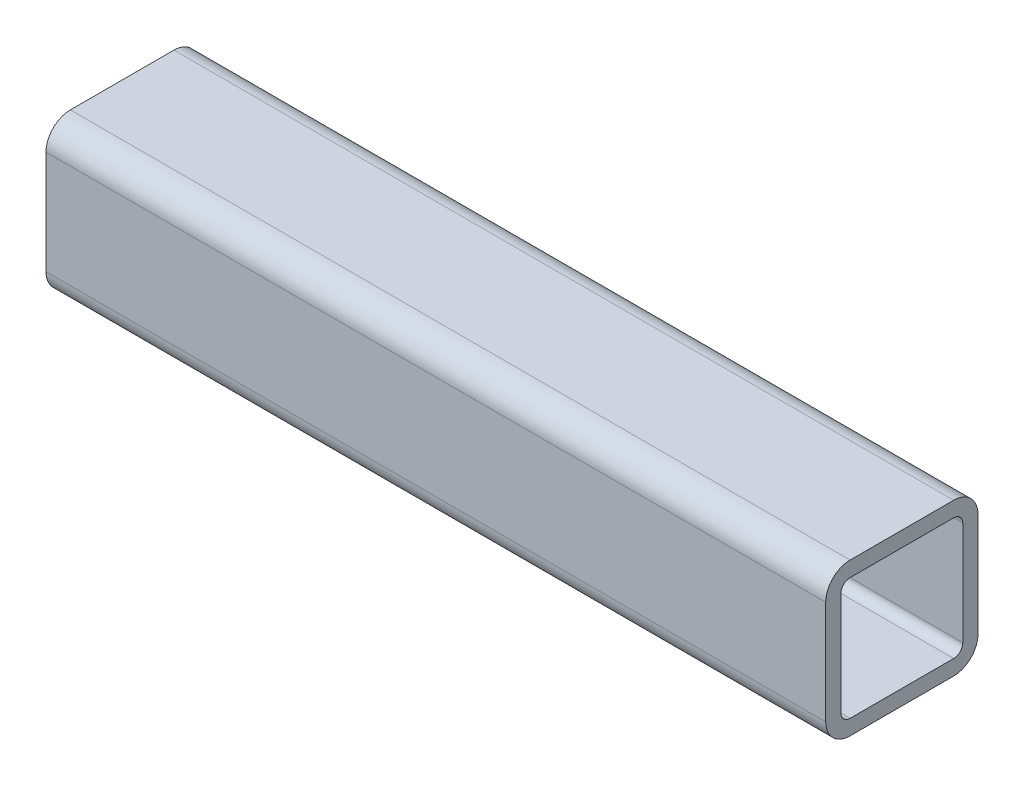
from build123d import *

# Parameters (mm, degrees)
COLD_FORMED_SQUARE_HOLLOW_SECTION_GB_T_6_DEPTH = 256


with BuildPart() as part:
    # Sketch1 → Cold-formed square hollow section GB/T 6728-2002 50 X 50 X 4(1) (new body)
    with BuildSketch(Plane.YZ.offset(-88.434077868)):
        with BuildLine():
            Line((-17, -25), (17, -25))
            ThreePointArc((17, -25), (22.656854249, -22.656854249), (25, -17))
            Line((25, -17), (25, 17))
            ThreePointArc((25, 17), (22.656854249, 22.656854249), (17, 25))
            Line((17, 25), (-17, 25))
            ThreePointArc((-17, 25), (-22.656854249, 22.656854249), (-25, 17))
            Line((-25, 17), (-25, -17))
            ThreePointArc((-25, -17), (-22.656854249, -22.656854249), (-17, -25))
        make_face()
        with BuildLine():
            Line((-17, -20), (17, -20))
            ThreePointArc((17, -20), (19.121320344, -19.121320344), (20, -17))
            Line((20, -17), (20, 17))
            ThreePointArc((20, 17), (19.121320344, 19.121320344), (17, 20))
            Line((17, 20), (-17, 20))
            ThreePointArc((-17, 20), (-19.121320344, 19.121320344), (-20, 17))
            Line((-20, 17), (-20, -17))
            ThreePointArc((-20, -17), (-19.121320344, -19.121320344), (-17, -20))
        make_face(mode=Mode.SUBTRACT)
    extrude(amount=COLD_FORMED_SQUARE_HOLLOW_SECTION_GB_T_6_DEPTH)


solid = part.part
